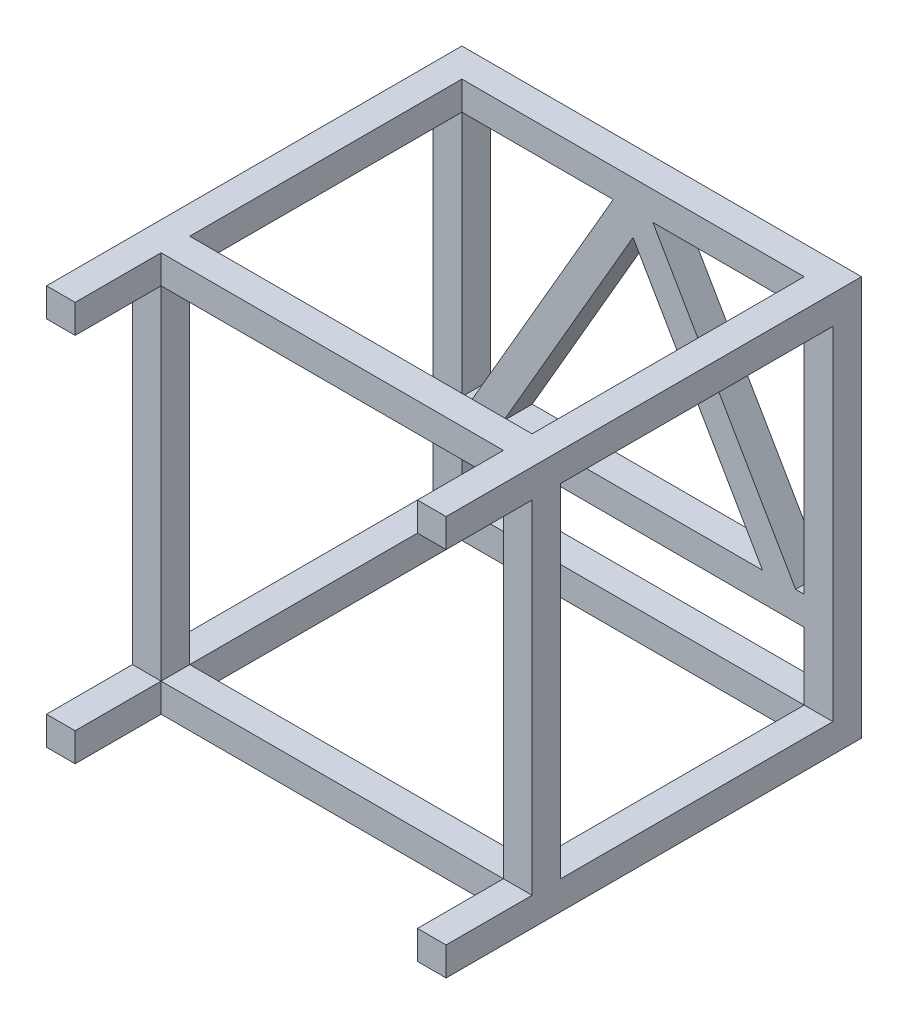
SolidWorks part; units mm, degrees
ref_plane "Front Plane" through (0, 0, 0) normal (0, 0, 1) x (1, 0, 0)
ref_plane "Top Plane" through (0, 0, 0) normal (0, 1, 0) x (1, 0, 0)
ref_plane "Right Plane" through (0, 0, 0) normal (1, 0, 0) x (0, 0, -1)
sketch "Sketch1" plane through (0, 0, 0) normal (0, 0, 1) x (1, 0, 0)
  line L0 (100, 100) -> (100, 335)
  line L1 (0, 0) -> (1395, 0)
  line L2 (0, 0) -> (0, 1395)
  line L3 (0, 1395) -> (1395, 1395)
  line L4 (1395, 0) -> (1395, 1395)
  line L5 (100, 1295) -> (628.2792, 1295)
  line L6 (1295, 100) -> (1295, 335)
  line L7 (100, 100) -> (1295, 100)
  line L8 (100, 335) -> (1295, 335)
  line L9 (100, 435) -> (130, 435)
  line L10 (766.7208, 1295) -> (1265, 435)
  line L11 (697.5, 1215) -> (1149.4276, 435)
  line L12 (697.5, 1215) -> (245.5724, 435)
  line L13 (628.2792, 1295) -> (130, 435)
  line L14 (245.5724, 435) -> (1149.4276, 435)
  line L15 (100, 435) -> (100, 1295)
  line L16 (100, 100) -> (100, 1295) construction
  line L17 (766.7208, 1295) -> (1295, 1295)
  line L18 (100, 1295) -> (1295, 1295) construction
  line L19 (1265, 435) -> (1295, 435)
  line L20 (1295, 435) -> (1295, 1295)
  line L21 (1295, 100) -> (1295, 1295) construction
  dimension "D1" = 1395
  dimension "D2" = 1395
  dimension "D4" = 235
  dimension "D5" = 100
  dimension "D6" = 100
  dimension "D7" = 100
  dimension "D8" = 30
  dimension "D9" = 30
  dimension "D10" = 697.5
  dimension "D11" = 80
  dimension "D3" = 100
extrude "Boss-Extrude1" add sketch "Sketch1" along normal blind 100
sketch "Sketch2" plane through (0, 0, 100) normal (0, 0, 1) x (1, 0, 0)
  line L1 (0, 1395) -> (100, 1395)
  line L2 (0, 1395) -> (0, 1295)
  line L3 (0, 1295) -> (100, 1295)
  line L4 (100, 1395) -> (100, 1295)
  line L5 (1395, 1395) -> (1295, 1395)
  line L6 (1395, 1395) -> (1395, 1295)
  line L7 (1395, 1295) -> (1295, 1295)
  line L8 (1295, 1395) -> (1295, 1295)
  line L9 (0, 0) -> (100, 0)
  line L10 (0, 0) -> (0, 100)
  line L11 (0, 100) -> (100, 100)
  line L12 (100, 0) -> (100, 100)
  line L13 (1395, 0) -> (1295, 0)
  line L14 (1395, 0) -> (1395, 100)
  line L15 (1395, 100) -> (1295, 100)
  line L16 (1295, 0) -> (1295, 100)
extrude "Boss-Extrude2" add sketch "Sketch2" along normal blind 1350
sketch "Sketch3" plane through (100, 0, 0) normal (1, 0, 0) x (0, 0, -1)
  line L0 (-1450, 0) -> (-100, 0) construction
  line L1 (-1050, 0) -> (-1150, 0)
  line L2 (-1050, 0) -> (-1050, 100)
  line L3 (-1050, 100) -> (-1150, 100)
  line L4 (-1150, 0) -> (-1150, 100)
  line L5 (-1450, 100) -> (-100, 100) construction
  line L6 (-1450, 0) -> (-1450, 100) construction
  line L7 (-1450, 1295) -> (-100, 1295) construction
  line L8 (-1050, 1295) -> (-1150, 1295)
  line L9 (-1050, 1295) -> (-1050, 1395)
  line L10 (-1050, 1395) -> (-1150, 1395)
  line L11 (-1150, 1295) -> (-1150, 1395)
  line L12 (-1450, 1395) -> (-100, 1395) construction
  dimension "D1" = 100
  dimension "D2" = 300
extrude "Boss-Extrude3" add sketch "Sketch3" along normal blind 1200
sketch "Sketch4" plane through (0, 100, 0) normal (0, 1, 0) x (1, 0, 0)
  line L0 (0, -1450) -> (0, -100) construction
  line L1 (100, -1050) -> (0, -1050)
  line L2 (100, -1050) -> (100, -1150)
  line L3 (100, -1150) -> (0, -1150)
  line L4 (0, -1050) -> (0, -1150)
  line L5 (1395, -1450) -> (1395, -100) construction
  line L6 (1295, -1050) -> (1395, -1050)
  line L7 (1295, -1050) -> (1295, -1150)
  line L8 (1295, -1150) -> (1395, -1150)
  line L9 (1395, -1050) -> (1395, -1150)
extrude "Boss-Extrude4" add sketch "Sketch4" along normal blind 1200
